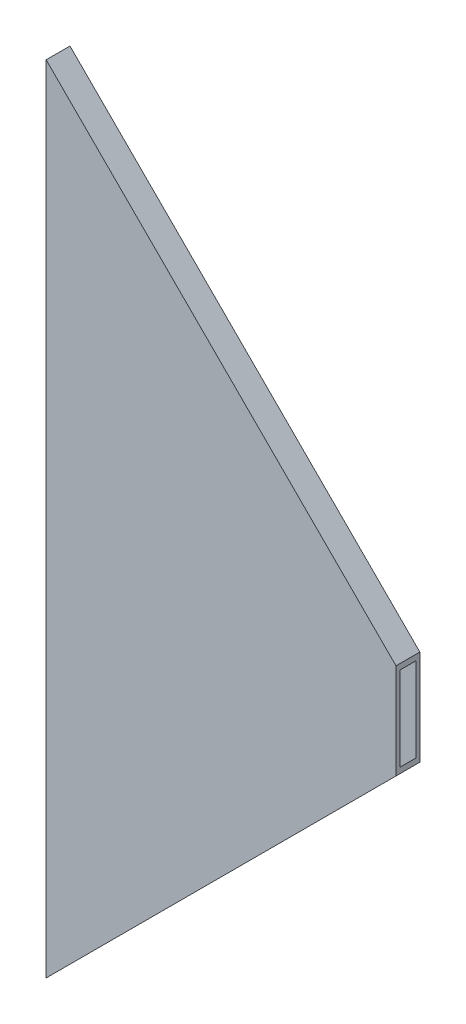
SolidWorks part; units mm, degrees
ref_plane "Front Plane" through (0, 0, 0) normal (0, 0, 1) x (1, 0, 0)
ref_plane "Top Plane" through (0, 0, 0) normal (0, 1, 0) x (1, 0, 0)
ref_plane "Right Plane" through (0, 0, 0) normal (1, 0, 0) x (0, 0, -1)
sketch "Sketch1" plane through (0, 0, 0) normal (0, 0, 1) x (1, 0, 0)
  line L0 (-500, 500) -> (0, 0)
  line L1 (-500, -500) -> (500, -500) construction
  line L2 (-500, -500) -> (-500, 500)
  line L3 (-500, 500) -> (500, 500) construction
  line L4 (500, -500) -> (500, 500) construction
  line L5 (-500, -500) -> (500, 500) construction
  line L6 (-500, 500) -> (500, -500) construction
  line L7 (0, 0) -> (-500, -500)
  point P0 (0, 0)
  dimension "D1" = 1000
extrude "Boss-Extrude1" add sketch "Sketch1" along normal blind 30
sketch "Sketch2" plane through (0, 0, 30) normal (0, 0, 1) x (1, 0, 0)
  line L0 (0, 0) -> (-500, 500) construction
  line L1 (60, -60) -> (-60, -60)
  line L2 (60, -60) -> (60, 60)
  line L3 (60, 60) -> (-60, 60)
  line L4 (-60, -60) -> (-60, 60)
  line L5 (60, -60) -> (-60, 60) construction
  line L6 (60, 60) -> (-60, -60) construction
  point P0 (0, 0)
  dimension "D1" = 120
extrude "Cut-Extrude1" cut sketch "Sketch2" against normal blind 30
sketch "Sketch3" plane through (-500, 0, 0) normal (-1, 0, 0) x (0, 0, 1)
  line L1 (25, 350) -> (-65, 350)
  line L2 (25, 350) -> (25, 300)
  line L3 (25, 300) -> (-65, 300)
  line L4 (-65, 350) -> (-65, 300)
  line L6 (7, 350) -> (-7, 350) construction
  line L7 (-7, 300) -> (7, 300) construction
  line L8 (0, 0) -> (-327.2098, 0) construction
  line L9 (-65, -350) -> (-65, -300)
  line L10 (25, -300) -> (-65, -300)
  line L11 (25, -350) -> (25, -300)
  line L12 (25, -350) -> (-65, -350)
  line L13 (30, 500) -> (30, -500) construction
  dimension "D1" = 90
  dimension "D2" = 5
extrude "Cut-Extrude2" cut sketch "Sketch3" against normal blind 7
shell "Shell1" thickness 5
hole_wizard "M4 Tapped Hole1" positions "Sketch4" profile "Sketch5" tap size "M4" standard "GB"
sketch "Sketch4" plane through (-493, 0, 0) normal (-1, 0, 0) x (0, 0, 1)
  point P0 (17.5, 335)
  point P3 (17.5, 315)
  point P6 (17.5, -315)
  point P9 (17.5, -335)
sketch "Sketch5" plane through (-493, 335, 17.5) normal (0, 1, 0) x (0, 0, 1)
  line L0 (0, 0) -> (0, 11.0914)
  line L1 (0, 11.0914) -> (1.65, 10.1)
  line L2 (1.65, 10.1) -> (1.65, 0)
  line L5 (1.65, 0) -> (0, 0)
  line L10 (0, 11.0914) -> (-1.65, 10.1) construction
  line L11 (0, -6.35) -> (0, 107.95) construction
  dimension "螺纹孔钻头直径" = 3.3
  dimension "螺纹孔钻头深度" = 10.1
  dimension "导头角度" = 118
cosmetic thread "Cosmetic thread 1" parameters "D1"=8, "D2"=4
cosmetic thread "Cosmetic thread 2" parameters "D1"=8, "D2"=4
cosmetic thread "Cosmetic thread 3" parameters "D1"=8, "D2"=4
cosmetic thread "Cosmetic thread 4" parameters "D1"=8, "D2"=4
